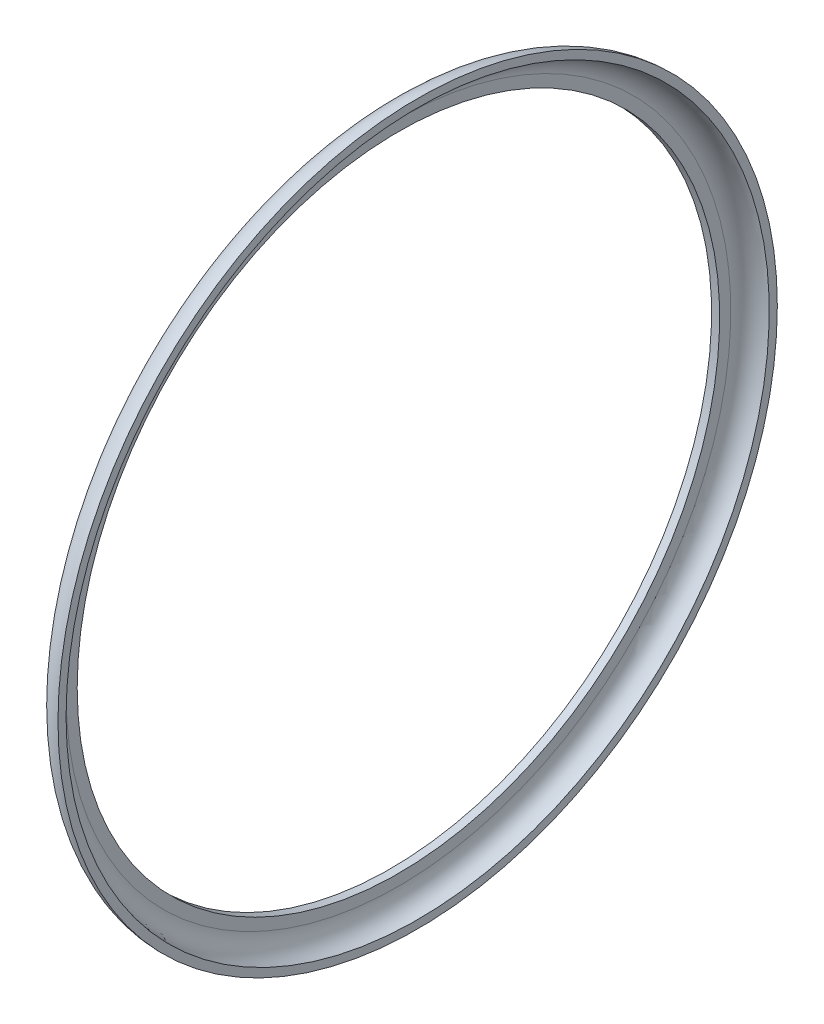
SolidWorks part; units mm, degrees
material "普通碳钢"
ref_plane "前视" through (0, 0, 0) normal (0, 0, 1) x (1, 0, 0)
ref_plane "上视" through (0, 0, 0) normal (0, 1, 0) x (1, 0, 0)
ref_plane "右视" through (0, 0, 0) normal (1, 0, 0) x (0, 0, -1)
sketch "草图1" plane through (0, 0, 0) normal (0, 0, 1) x (1, 0, 0)
  line L0 (-257.7667, 0) -> (287.5333, 0) construction
  line L1 (0, 204.25) -> (0, -166.8833) construction
  line L2 (-27, 328.5) -> (-27, 317.5)
  line L4 (-19, 328.5) -> (-19, 317.5)
  line L5 (0, 355.5) -> (0, 347.5)
  line L6 (-27, 317.5) -> (-19, 317.5)
  arc A0 (0, 347.5) -> (-19, 328.5) centre (0, 328.5) ccw
  arc A1 (0, 355.5) -> (-27, 328.5) centre (0, 328.5) ccw
  dimension "D1" = 38
  dimension "D2" = 54
  dimension "D3" = 328.5
  dimension "D4" = 11
revolve "旋转1" add sketch "草图1" angle 360 about L0
